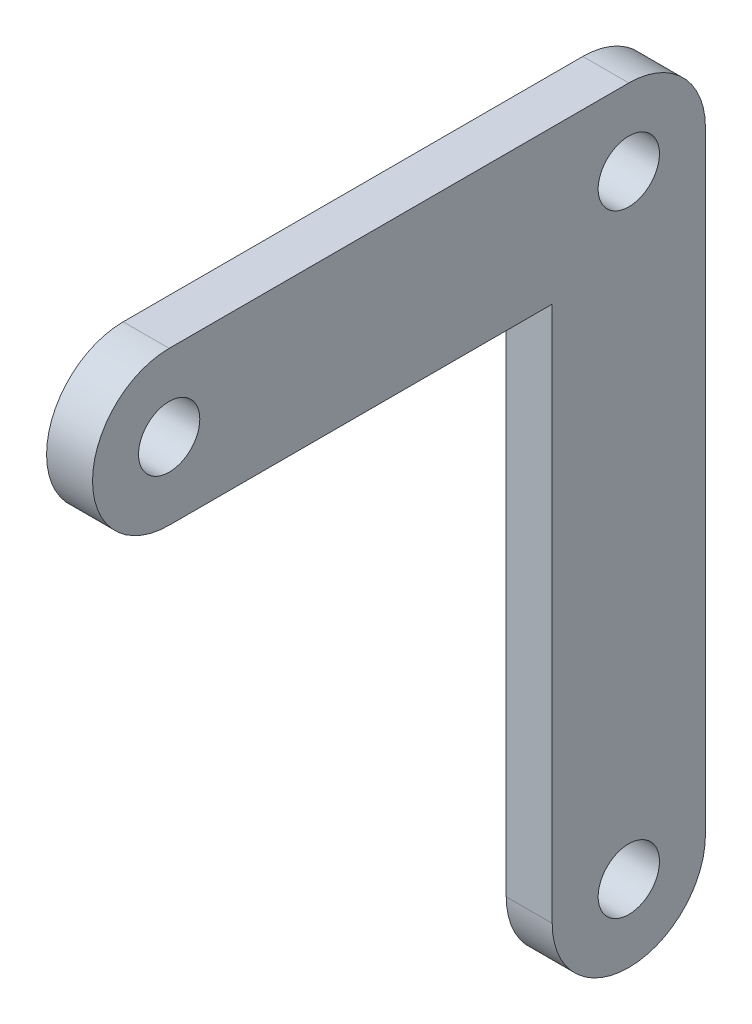
from build123d import *

# Parameters (mm, degrees)
SKETCH1_R           = 4
BOSS_EXTRUDE1_DEPTH = 6


with BuildPart() as part:
    # Sketch1 → Boss-Extrude1 (new body)
    # profile 1 of 3: a face of its own
    with BuildSketch(Plane(origin=(0, 0, 0), x_dir=(0, 0, -1), z_dir=(1, 0, 0))):
        with BuildLine():
            Line((60, 10), (0, 10))
            ThreePointArc((0, 10), (-10, 0), (0, -10))
            Line((0, -10), (50, -10))
            Line((50, -10), (50, 0))
            ThreePointArc((50, 0), (52.928932188, 7.071067812), (60, 10))
        make_face()
        Circle(SKETCH1_R, mode=Mode.SUBTRACT)
    # profile 2 of 3: a face of its own
    with BuildSketch(Plane(origin=(0, 0, 0), x_dir=(0, 0, -1), z_dir=(1, 0, 0))):
        with BuildLine():
            ThreePointArc((70, 0), (67.071067812, 7.071067812), (60, 10))
            ThreePointArc((60, 10), (52.928932188, 7.071067812), (50, 0))
            Line((50, 0), (50, -10))
            Line((50, -10), (60, -10))
            ThreePointArc((60, -10), (67.071067812, -7.071067812), (70, 0))
        make_face()
        with Locations((60, 0)):
            Circle(SKETCH1_R, mode=Mode.SUBTRACT)
    # profile 3 of 3: a face of its own
    with BuildSketch(Plane(origin=(0, 0, 0), x_dir=(0, 0, -1), z_dir=(1, 0, 0))):
        with BuildLine():
            Line((70, -80), (70, 0))
            ThreePointArc((70, 0), (67.071067812, -7.071067812), (60, -10))
            Line((60, -10), (50, -10))
            Line((50, -10), (50, -80))
            ThreePointArc((50, -80), (60, -90), (70, -80))
        make_face()
        with Locations((60, -80)):
            Circle(SKETCH1_R, mode=Mode.SUBTRACT)
    extrude(amount=BOSS_EXTRUDE1_DEPTH)


solid = part.part
